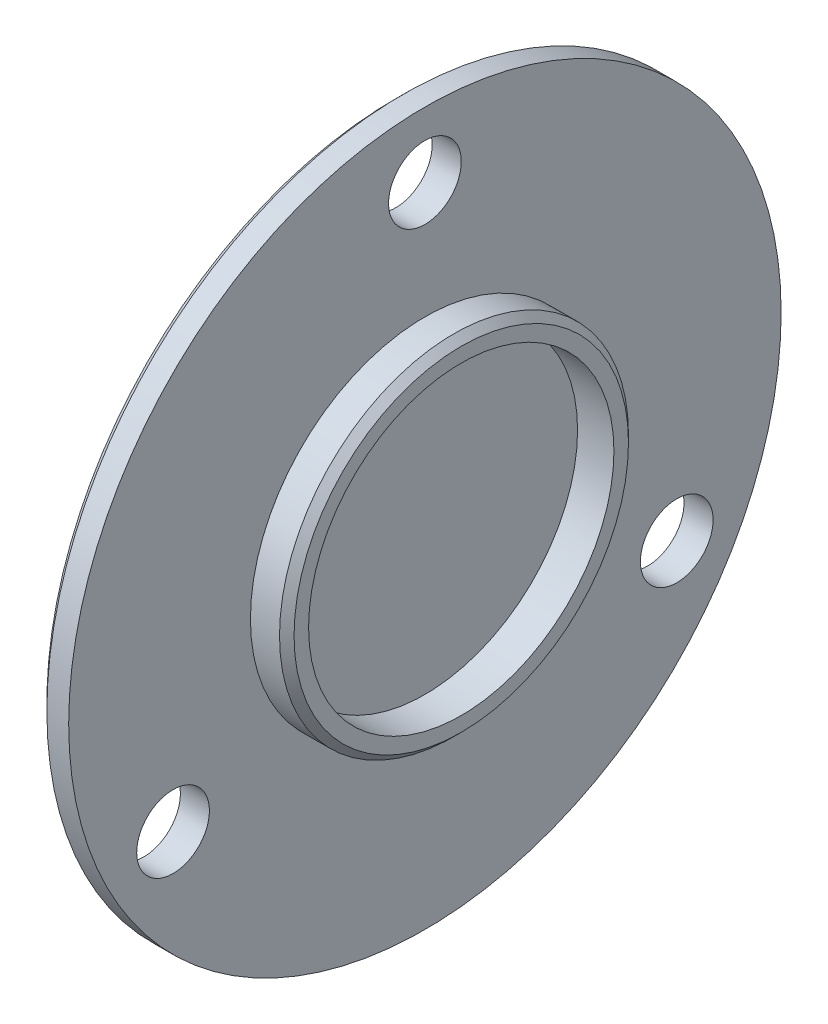
SolidWorks part; units mm, degrees
ref_plane "Front Plane" through (0, 0, 0) normal (0, 0, 1) x (1, 0, 0)
ref_plane "Top Plane" through (0, 0, 0) normal (0, 1, 0) x (1, 0, 0)
ref_plane "Right Plane" through (0, 0, 0) normal (1, 0, 0) x (0, 0, -1)
other "Configuration Table"
sketch "Sketch1" plane through (0, 0, 0) normal (1, 0, 0) x (0, 0, -1)
  circle A1 centre (0, 0) radius 24.5
  dimension "D1" = 49
extrude "Boss-Extrude1" add sketch "Sketch1" along normal blind 2
sketch "Sketch2" plane through (2, 0, 0) normal (1, 0, 0) x (0, 0, -1)
  circle A0 centre (0, 0) radius 12
  dimension "D1" = 24
extrude "Boss-Extrude2" add sketch "Sketch2" along normal blind 2.5
sketch "Sketch3" plane through (4.5, 0, 0) normal (1, 0, 0) x (0, 0, -1)
  circle A0 centre (0, 0) radius 10.5
  dimension "D1" = 21
extrude "Cut-Extrude1" cut sketch "Sketch3" against normal blind 2.5 and the other way through all
sketch "Sketch4" plane through (0, 0, 0) normal (-1, 0, 0) x (0, 0, 1)
  line L0 (0, 20) -> (0, 0) construction
  circle A0 centre (0, 20) radius 2.5
  circle A1 centre (17.3205, -10) radius 2.5
  circle A2 centre (-17.3205, -10) radius 2.5
  point P11 (0, 0)
  dimension "D1" = 5
  dimension "D2" = 20
  dimension "D3" = 3
extrude "Cut-Extrude2" cut sketch "Sketch4" against normal blind 2.5
chamfer "Chamfer1" distance 0.5 angle 45 2 edges at (0, 0, -24.5) (4.5, 0, -12)
